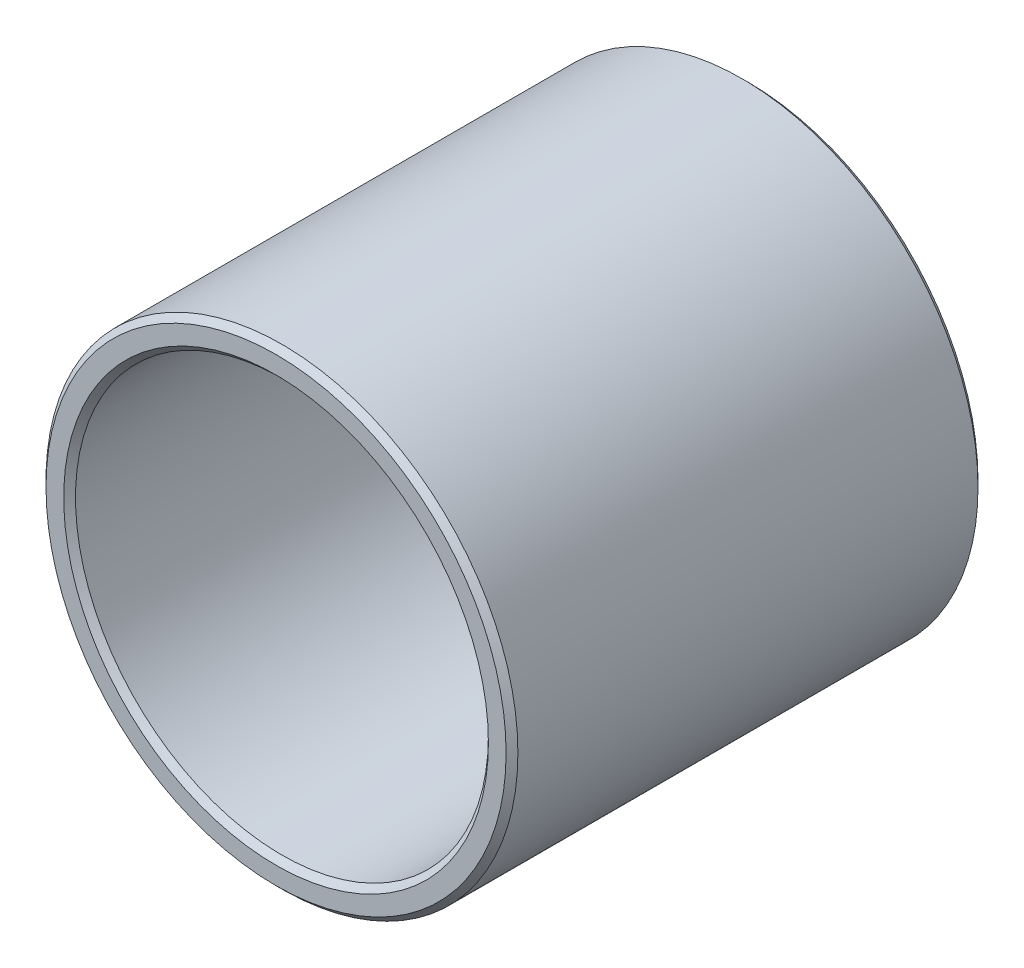
from build123d import *

# Parameters (mm, degrees)
SKETCH1_R           = 40
SKETCH1_R_2         = 35
BOSS_EXTRUDE1_DEPTH = 40
CHAMFER1_SIZE       = 1


with BuildPart() as part:
    # Sketch1 → Boss-Extrude1 (new, symmetric)
    with BuildSketch(Plane.XY):
        Circle(SKETCH1_R)
        Circle(SKETCH1_R_2, mode=Mode.SUBTRACT)
    extrude(amount=BOSS_EXTRUDE1_DEPTH, both=True)

    # Chamfer1
    chamfer1_edges = [part.edges().sort_by_distance(p)[0] for p in [
        (-40, 0, -40),
        (-40, 0, 40),
        (-35, 0, -40),
        (-35, 0, 40),
    ]]
    chamfer(chamfer1_edges, length=CHAMFER1_SIZE)


solid = part.part
